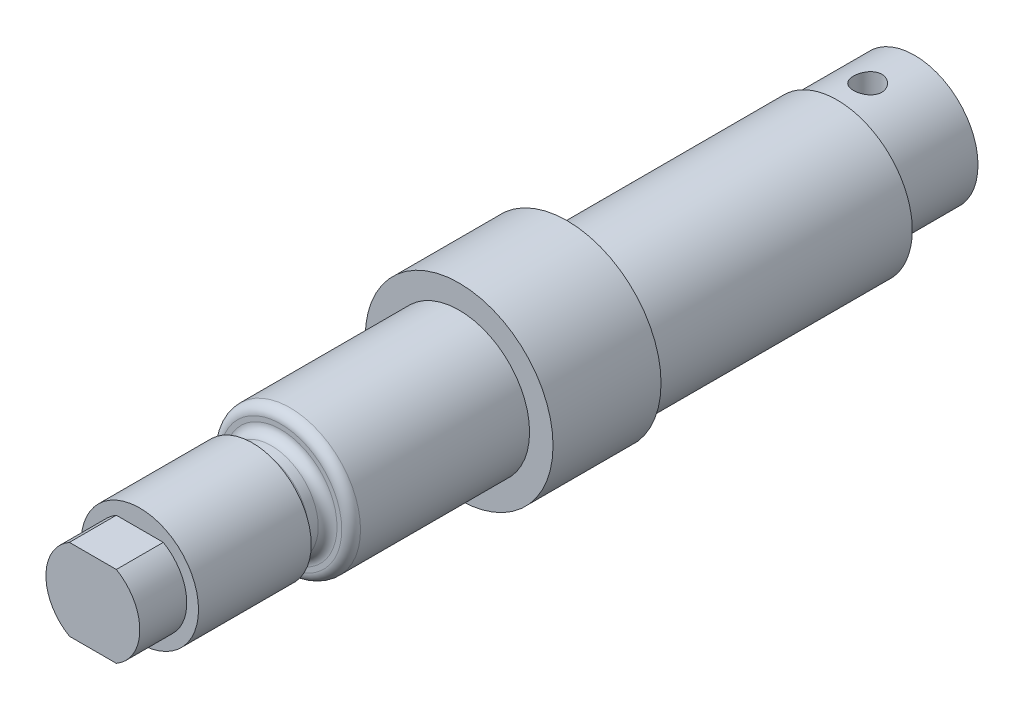
from build123d import *

# Parameters (mm, degrees)
SKETCH2_R          = 13.5
EXTRUDE1_DEPTH     = 19
SKETCH3_R          = 16
EXTRUDE2_DEPTH     = 55
SKETCH4_R          = 20
EXTRUDE3_DEPTH     = 23
SKETCH5_R          = 15
EXTRUDE4_DEPTH     = 38
SKETCH6_R          = 10
EXTRUDE5_DEPTH     = 6
SKETCH7_R          = 12.5
EXTRUDE6_DEPTH     = 24
EXTRUDE7_DEPTH     = 10
SKETCH9_R          = 3
CUT_EXTRUDE1_DEPTH = 15
FILLET1_R          = 2


with BuildPart() as part:
    # Sketch2 → Extrude1 (new body)
    with BuildSketch(Plane.XY):
        Circle(SKETCH2_R)
    extrude(amount=EXTRUDE1_DEPTH)

    # Sketch3 → Extrude2 (add)
    with BuildSketch(Plane.XY.offset(19)):
        with Locations(Location((2.5, 0, 0), (0, 0, 179.999529266))):
            Circle(SKETCH3_R)
    extrude(amount=EXTRUDE2_DEPTH)

    # Sketch4 → Extrude3 (add)
    with BuildSketch(Plane.XY.offset(74)):
        Circle(SKETCH4_R)
    extrude(amount=EXTRUDE3_DEPTH)

    # Sketch5 → Extrude4 (add)
    with BuildSketch(Plane.XY.offset(97)):
        Circle(SKETCH5_R)
    extrude(amount=EXTRUDE4_DEPTH)

    # Sketch6 → Extrude5 (add)
    with BuildSketch(Plane.XY.offset(135)):
        Circle(SKETCH6_R)
    extrude(amount=EXTRUDE5_DEPTH)

    # Sketch7 → Extrude6 (add)
    with BuildSketch(Plane.XY.offset(141)):
        Circle(SKETCH7_R)
    extrude(amount=EXTRUDE6_DEPTH)

    # Sketch8 → Extrude7 (add)
    with BuildSketch(Plane.XY.offset(165)):
        with BuildLine():
            Line((-5, 8.660254038), (5, 8.660254038))
            ThreePointArc((5, 8.660254038), (10, 0), (5, -8.660254038))
            Line((5, -8.660254038), (-5, -8.660254038))
            ThreePointArc((-5, -8.660254038), (-10, 0), (-5, 8.660254038))
        make_face()
    extrude(amount=EXTRUDE7_DEPTH)

    # Sketch9 → Cut-Extrude1 (cut, symmetric)
    with BuildSketch(Plane(origin=(0, 0, 0), x_dir=(1, 0, 0), z_dir=(0, 1, 0))):
        with Locations(Location((0, -10, 0), (0, 0, 270))):
            Circle(SKETCH9_R)
    extrude(amount=CUT_EXTRUDE1_DEPTH, both=True, mode=Mode.SUBTRACT)

    # Fillet1
    fillet1_edges = [part.edges().sort_by_distance(p)[0] for p in [
        (-15, 0, 135),
        (-10, 0, 135),
        (-10, 0, 141),
    ]]
    fillet(fillet1_edges, radius=FILLET1_R)


solid = part.part
